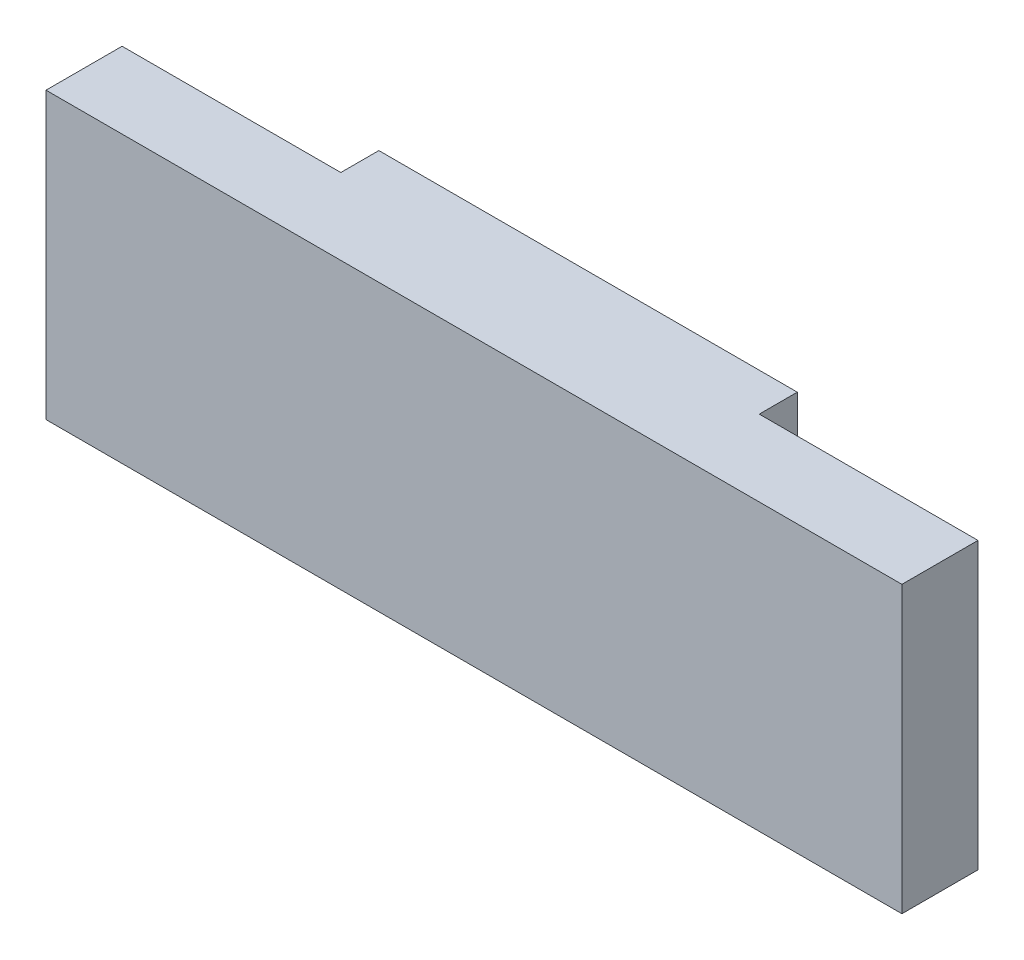
SolidWorks part; units mm, degrees
ref_plane "Front Plane" through (0, 0, 0) normal (0, 0, 1) x (1, 0, 0)
ref_plane "Top Plane" through (0, 0, 0) normal (0, 1, 0) x (1, 0, 0)
ref_plane "Right Plane" through (0, 0, 0) normal (1, 0, 0) x (0, 0, -1)
sketch "Sketch1" plane through (0, 0, 0) normal (0, 1, 0) x (1, 0, 0)
  line L0 (115, 0) -> (115, 20)
  line L1 (0, 0) -> (115, 0)
  line L2 (0, 0) -> (0, -40)
  line L3 (0, -40) -> (450, -40)
  line L4 (450, 0) -> (450, -40)
  line L5 (115, 20) -> (335, 20)
  line L6 (335, 20) -> (335, 0)
  line L7 (335, 0) -> (450, 0)
  line L8 (225, 20) -> (225, -40) construction
  dimension "D1" = 450
  dimension "D2" = 40
  dimension "D3" = 220
  dimension "D4" = 20
extrude "Boss-Extrude1" add sketch "Sketch1" along normal blind 150
